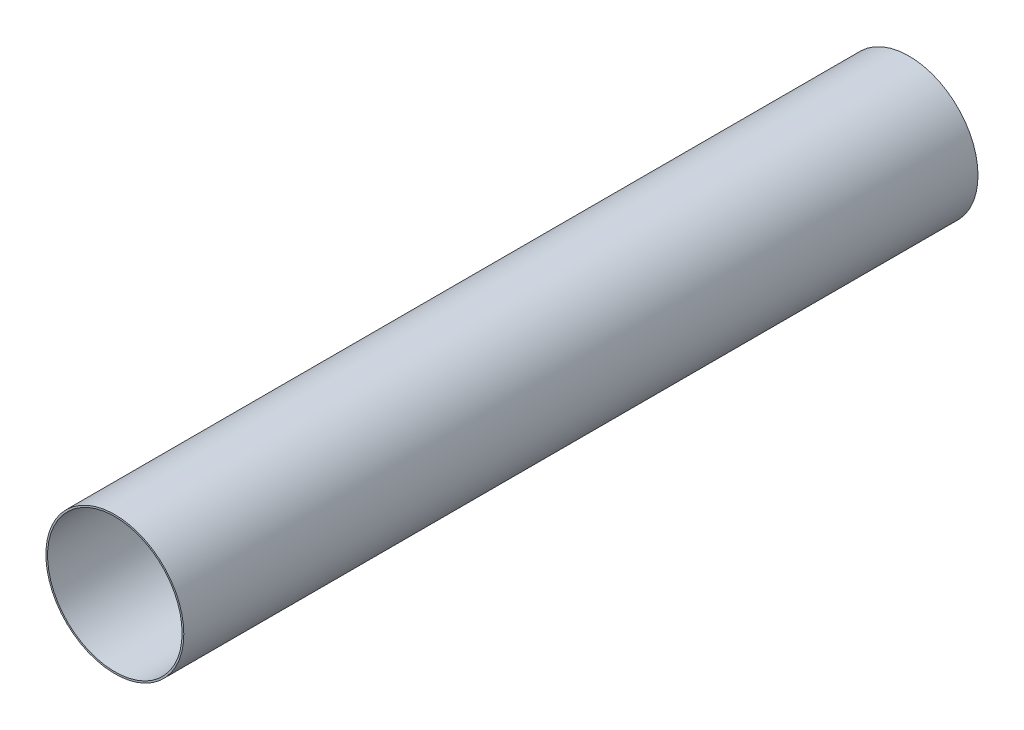
SolidWorks part; units mm, degrees
ref_plane "前视基准面" through (0, 0, 0) normal (0, 0, 1) x (1, 0, 0)
ref_plane "上视基准面" through (0, 0, 0) normal (0, 1, 0) x (1, 0, 0)
ref_plane "右视基准面" through (0, 0, 0) normal (1, 0, 0) x (0, 0, -1)
other "Configuration Table"
sketch "草图1" plane through (0, 0, 0) normal (0, 0, 1) x (1, 0, 0)
  circle A0 centre (0, 0) radius 48.5
  circle A1 centre (0, 0) radius 47.3
  dimension "D1" = 97
  dimension "D2" = 94.6
extrude "凸台-拉伸1" add sketch "草图1" along normal blind 558.5
